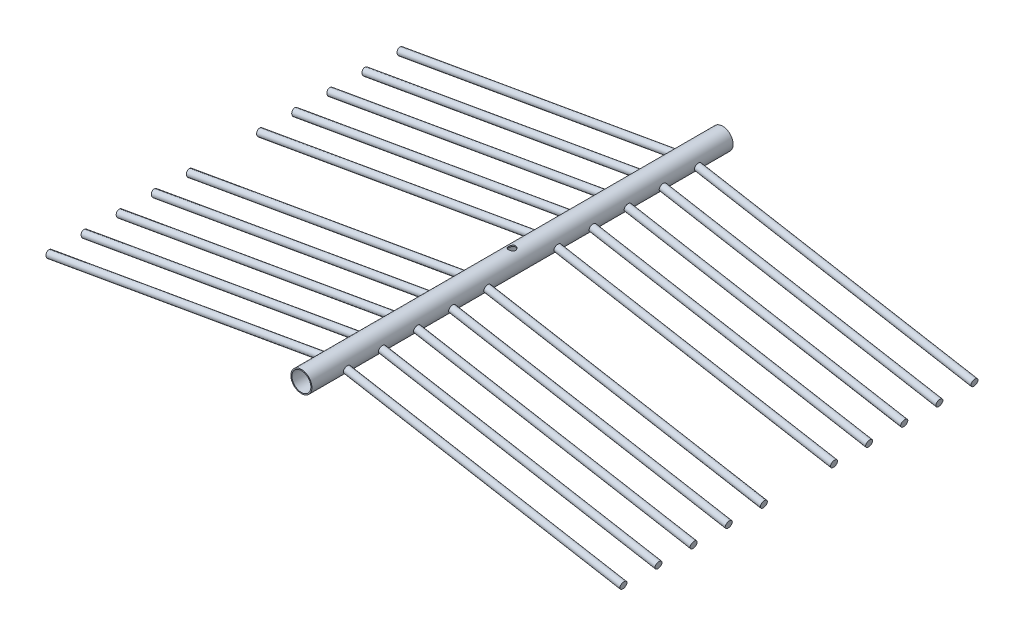
from build123d import *

# Parameters (mm, degrees)
SKETCH1_R              = 15
BOSS_EXTRUDE1_DEPTH    = 600
SKETCH5_R              = 5
BOSS_EXTRUDE3_DEPTH    = 400
BOSS_EXTRUDE3_2_DEPTH  = 400
BOSS_EXTRUDE3_3_DEPTH  = 400
BOSS_EXTRUDE3_4_DEPTH  = 400
BOSS_EXTRUDE3_5_DEPTH  = 400
BOSS_EXTRUDE3_6_DEPTH  = 400
BOSS_EXTRUDE3_7_DEPTH  = 400
BOSS_EXTRUDE3_8_DEPTH  = 400
BOSS_EXTRUDE3_9_DEPTH  = 400
BOSS_EXTRUDE3_10_DEPTH = 400
SKETCH6_R              = 5
BOSS_EXTRUDE4_DEPTH    = 400
BOSS_EXTRUDE4_2_DEPTH  = 400
BOSS_EXTRUDE4_3_DEPTH  = 400
BOSS_EXTRUDE4_4_DEPTH  = 400
BOSS_EXTRUDE4_5_DEPTH  = 400
BOSS_EXTRUDE4_6_DEPTH  = 400
BOSS_EXTRUDE4_7_DEPTH  = 400
BOSS_EXTRUDE4_8_DEPTH  = 400
BOSS_EXTRUDE4_9_DEPTH  = 400
BOSS_EXTRUDE4_10_DEPTH = 400
SKETCH7_R              = 5
CUT_EXTRUDE1_DEPTH     = 731.526784995
SKETCH8_R              = 13.5
CUT_EXTRUDE2_DEPTH     = 731.526785077


with BuildPart() as part:
    # Sketch1 → Boss-Extrude1 (new body)
    with BuildSketch(Plane.XY):
        Circle(SKETCH1_R)
    extrude(amount=BOSS_EXTRUDE1_DEPTH)

    # Sketch7 → Cut-Extrude1 (cut, through all)
    with BuildSketch(Plane(origin=(0, 0, 0), x_dir=(1, 0, 0), z_dir=(0, 1, 0))):
        with Locations(Location((0, -300, 0), (0, 0, 90))):
            Circle(SKETCH7_R)
    extrude(amount=CUT_EXTRUDE1_DEPTH, mode=Mode.SUBTRACT)

    # Sketch8 → Cut-Extrude2 (cut, through all)
    with BuildSketch(Plane.XY.offset(600)):
        Circle(SKETCH8_R)
    extrude(amount=-CUT_EXTRUDE2_DEPTH, mode=Mode.SUBTRACT)


with BuildPart() as body_2:
    # Sketch5 → Boss-Extrude3 (new body)
    with BuildSketch(Plane(origin=(-14.772116295, -2.604722665, 0), x_dir=(0, 0, -1), z_dir=(-0.9848077530122086, -0.17364817766692736, 0))):
        with Locations(Location((-350, 0, 0), (0, 0, 90))):
            Circle(SKETCH5_R)
    extrude(amount=BOSS_EXTRUDE3_DEPTH)


with BuildPart() as body_3:
    # Sketch5 → Boss-Extrude3 2 (new body)
    with BuildSketch(Plane(origin=(-14.772116295, -2.604722665, 0), x_dir=(0, 0, -1), z_dir=(-0.9848077530122086, -0.17364817766692736, 0))):
        with Locations(Location((-400, 0, 0), (0, 0, 90))):
            Circle(SKETCH5_R)
    extrude(amount=BOSS_EXTRUDE3_2_DEPTH)


with BuildPart() as body_4:
    # Sketch5 → Boss-Extrude3 3 (new body)
    with BuildSketch(Plane(origin=(-14.772116295, -2.604722665, 0), x_dir=(0, 0, -1), z_dir=(-0.9848077530122086, -0.17364817766692736, 0))):
        with Locations(Location((-450, 0, 0), (0, 0, 90))):
            Circle(SKETCH5_R)
    extrude(amount=BOSS_EXTRUDE3_3_DEPTH)


with BuildPart() as body_5:
    # Sketch5 → Boss-Extrude3 4 (new body)
    with BuildSketch(Plane(origin=(-14.772116295, -2.604722665, 0), x_dir=(0, 0, -1), z_dir=(-0.9848077530122086, -0.17364817766692736, 0))):
        with Locations(Location((-500, 0, 0), (0, 0, 90))):
            Circle(SKETCH5_R)
    extrude(amount=BOSS_EXTRUDE3_4_DEPTH)


with BuildPart() as body_6:
    # Sketch5 → Boss-Extrude3 5 (new body)
    with BuildSketch(Plane(origin=(-14.772116295, -2.604722665, 0), x_dir=(0, 0, -1), z_dir=(-0.9848077530122086, -0.17364817766692736, 0))):
        with Locations(Location((-550, 0, 0), (0, 0, 90))):
            Circle(SKETCH5_R)
    extrude(amount=BOSS_EXTRUDE3_5_DEPTH)


with BuildPart() as body_7:
    # Sketch5 → Boss-Extrude3 6 (new body)
    with BuildSketch(Plane(origin=(-14.772116295, -2.604722665, 0), x_dir=(0, 0, -1), z_dir=(-0.9848077530122086, -0.17364817766692736, 0))):
        with Locations(Location((-250, 0, 0), (0, 0, 270))):
            Circle(SKETCH5_R)
    extrude(amount=BOSS_EXTRUDE3_6_DEPTH)


with BuildPart() as body_8:
    # Sketch5 → Boss-Extrude3 7 (new body)
    with BuildSketch(Plane(origin=(-14.772116295, -2.604722665, 0), x_dir=(0, 0, -1), z_dir=(-0.9848077530122086, -0.17364817766692736, 0))):
        with Locations(Location((-200, 0, 0), (0, 0, 270))):
            Circle(SKETCH5_R)
    extrude(amount=BOSS_EXTRUDE3_7_DEPTH)


with BuildPart() as body_9:
    # Sketch5 → Boss-Extrude3 8 (new body)
    with BuildSketch(Plane(origin=(-14.772116295, -2.604722665, 0), x_dir=(0, 0, -1), z_dir=(-0.9848077530122086, -0.17364817766692736, 0))):
        with Locations(Location((-150, 0, 0), (0, 0, 270))):
            Circle(SKETCH5_R)
    extrude(amount=BOSS_EXTRUDE3_8_DEPTH)


with BuildPart() as body_10:
    # Sketch5 → Boss-Extrude3 9 (new body)
    with BuildSketch(Plane(origin=(-14.772116295, -2.604722665, 0), x_dir=(0, 0, -1), z_dir=(-0.9848077530122086, -0.17364817766692736, 0))):
        with Locations(Location((-100, 0, 0), (0, 0, 270))):
            Circle(SKETCH5_R)
    extrude(amount=BOSS_EXTRUDE3_9_DEPTH)


with BuildPart() as body_11:
    # Sketch5 → Boss-Extrude3 10 (new body)
    with BuildSketch(Plane(origin=(-14.772116295, -2.604722665, 0), x_dir=(0, 0, -1), z_dir=(-0.9848077530122086, -0.17364817766692736, 0))):
        with Locations(Location((-50, 0, 0), (0, 0, 270))):
            Circle(SKETCH5_R)
    extrude(amount=BOSS_EXTRUDE3_10_DEPTH)


with BuildPart() as body_12:
    # Sketch6 → Boss-Extrude4 (new body)
    with BuildSketch(Plane(origin=(14.772116295, -2.604722665, 0), x_dir=(0, 0, -1), z_dir=(0.9848077530122075, -0.17364817766693402, 0))):
        with Locations(Location((-550, 0, 0), (0, 0, 90))):
            Circle(SKETCH6_R)
    extrude(amount=BOSS_EXTRUDE4_DEPTH)


with BuildPart() as body_13:
    # Sketch6 → Boss-Extrude4 2 (new body)
    with BuildSketch(Plane(origin=(14.772116295, -2.604722665, 0), x_dir=(0, 0, -1), z_dir=(0.9848077530122075, -0.17364817766693402, 0))):
        with Locations(Location((-500, 0, 0), (0, 0, 90))):
            Circle(SKETCH6_R)
    extrude(amount=BOSS_EXTRUDE4_2_DEPTH)


with BuildPart() as body_14:
    # Sketch6 → Boss-Extrude4 3 (new body)
    with BuildSketch(Plane(origin=(14.772116295, -2.604722665, 0), x_dir=(0, 0, -1), z_dir=(0.9848077530122075, -0.17364817766693402, 0))):
        with Locations(Location((-450, 0, 0), (0, 0, 90))):
            Circle(SKETCH6_R)
    extrude(amount=BOSS_EXTRUDE4_3_DEPTH)


with BuildPart() as body_15:
    # Sketch6 → Boss-Extrude4 4 (new body)
    with BuildSketch(Plane(origin=(14.772116295, -2.604722665, 0), x_dir=(0, 0, -1), z_dir=(0.9848077530122075, -0.17364817766693402, 0))):
        with Locations(Location((-400, 0, 0), (0, 0, 90))):
            Circle(SKETCH6_R)
    extrude(amount=BOSS_EXTRUDE4_4_DEPTH)


with BuildPart() as body_16:
    # Sketch6 → Boss-Extrude4 5 (new body)
    with BuildSketch(Plane(origin=(14.772116295, -2.604722665, 0), x_dir=(0, 0, -1), z_dir=(0.9848077530122075, -0.17364817766693402, 0))):
        with Locations(Location((-350, 0, 0), (0, 0, 90))):
            Circle(SKETCH6_R)
    extrude(amount=BOSS_EXTRUDE4_5_DEPTH)


with BuildPart() as body_17:
    # Sketch6 → Boss-Extrude4 6 (new body)
    with BuildSketch(Plane(origin=(14.772116295, -2.604722665, 0), x_dir=(0, 0, -1), z_dir=(0.9848077530122075, -0.17364817766693402, 0))):
        with Locations(Location((-250, 0, 0), (0, 0, 270))):
            Circle(SKETCH6_R)
    extrude(amount=BOSS_EXTRUDE4_6_DEPTH)


with BuildPart() as body_18:
    # Sketch6 → Boss-Extrude4 7 (new body)
    with BuildSketch(Plane(origin=(14.772116295, -2.604722665, 0), x_dir=(0, 0, -1), z_dir=(0.9848077530122075, -0.17364817766693402, 0))):
        with Locations(Location((-200, 0, 0), (0, 0, 270))):
            Circle(SKETCH6_R)
    extrude(amount=BOSS_EXTRUDE4_7_DEPTH)


with BuildPart() as body_19:
    # Sketch6 → Boss-Extrude4 8 (new body)
    with BuildSketch(Plane(origin=(14.772116295, -2.604722665, 0), x_dir=(0, 0, -1), z_dir=(0.9848077530122075, -0.17364817766693402, 0))):
        with Locations(Location((-150, 0, 0), (0, 0, 270))):
            Circle(SKETCH6_R)
    extrude(amount=BOSS_EXTRUDE4_8_DEPTH)


with BuildPart() as body_20:
    # Sketch6 → Boss-Extrude4 9 (new body)
    with BuildSketch(Plane(origin=(14.772116295, -2.604722665, 0), x_dir=(0, 0, -1), z_dir=(0.9848077530122075, -0.17364817766693402, 0))):
        with Locations(Location((-100, 0, 0), (0, 0, 270))):
            Circle(SKETCH6_R)
    extrude(amount=BOSS_EXTRUDE4_9_DEPTH)


with BuildPart() as body_21:
    # Sketch6 → Boss-Extrude4 10 (new body)
    with BuildSketch(Plane(origin=(14.772116295, -2.604722665, 0), x_dir=(0, 0, -1), z_dir=(0.9848077530122075, -0.17364817766693402, 0))):
        with Locations(Location((-50, 0, 0), (0, 0, 270))):
            Circle(SKETCH6_R)
    extrude(amount=BOSS_EXTRUDE4_10_DEPTH)


solid = Compound([part.part, body_2.part, body_3.part, body_4.part, body_5.part, body_6.part, body_7.part, body_8.part, body_9.part, body_10.part, body_11.part, body_12.part, body_13.part, body_14.part, body_15.part, body_16.part, body_17.part, body_18.part, body_19.part, body_20.part, body_21.part])
